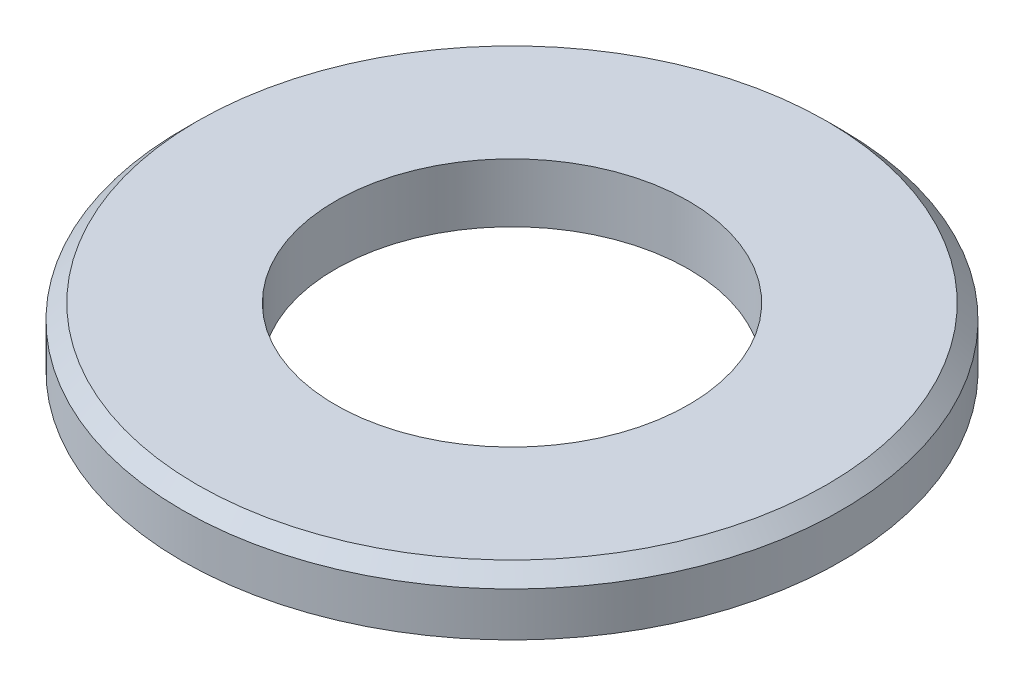
from build123d import *


with BuildPart() as part:
    # Sketch1 → Base-Revolve (revolve)
    with BuildSketch(Plane.XY, mode=Mode.PRIVATE) as base_revolve_sk:
        Polygon((-13.375, 11.144507042), (-14, 10.519507042), (-14, 8.644507042), (-7.5, 8.644507042), (-7.5, 11.144507042), align=None)
    revolve(base_revolve_sk.sketch.rotate(Axis((0, 0, 0), (0, 1, 0)), 270), axis=Axis((0, 0, 0), (0, 1, 0)))


solid = part.part
